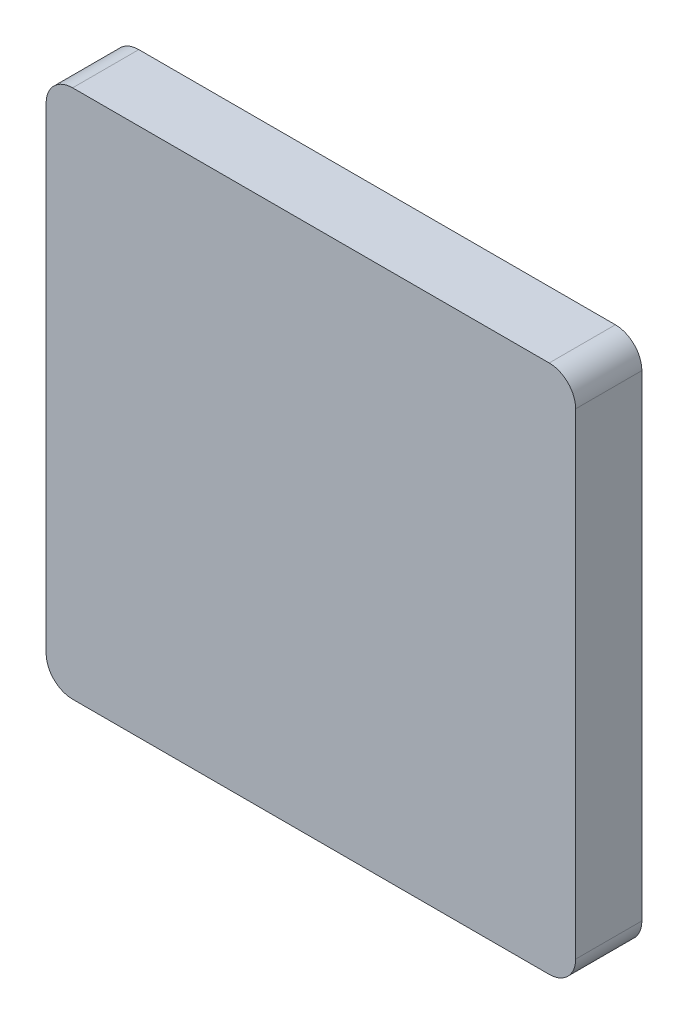
from build123d import *

# Parameters (mm, degrees)
BOSS_EXTRUDE1_DEPTH = 5


with BuildPart() as part:
    # Sketch1 → Boss-Extrude1 (new body)
    with BuildSketch(Plane.XY):
        with BuildLine():
            Line((2, 0), (38, 0))
            ThreePointArc((38, 0), (39.414213562, 0.585786438), (40, 2))
            Line((40, 2), (40, 38))
            ThreePointArc((40, 38), (39.414213562, 39.414213562), (38, 40))
            Line((38, 40), (2, 40))
            ThreePointArc((2, 40), (0.585786438, 39.414213562), (0, 38))
            Line((0, 38), (0, 2))
            ThreePointArc((0, 2), (0.585786438, 0.585786438), (2, 0))
        make_face()
    extrude(amount=BOSS_EXTRUDE1_DEPTH)


solid = part.part
